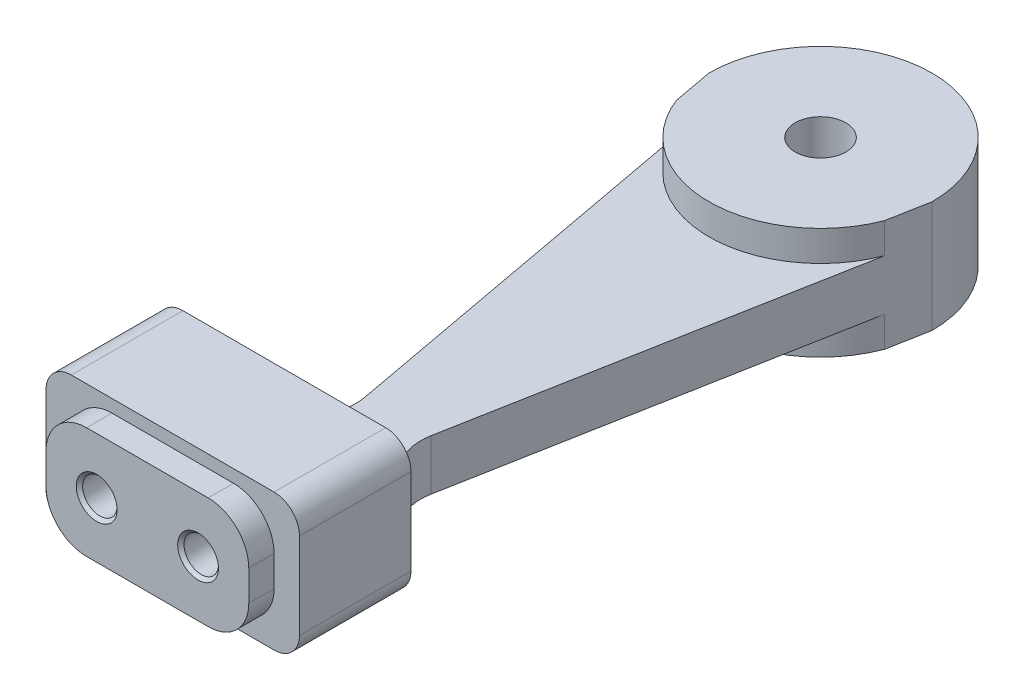
from build123d import *

# Parameters (mm, degrees)
BOSS_EXTRUDE1_DEPTH         = 22
BOSS_EXTRUDE2_DEPTH         = 5
BOSS_EXTRUDE3_DEPTH         = 5
SKETCH_4_3_2_R              = 5
BOSS_EXTRUDE4_DEPTH         = 11
M8_TAPPED_HOLE1_D           = 6.8
M8_TAPPED_HOLE1_DEPTH       = 19.957073895
M8_TAPPED_HOLE1_CSINK_D     = 8.05
M8_TAPPED_HOLE1_CSINK_ANGLE = 90
M8_TAPPED_HOLE1_TIP         = 2.042926105


with BuildPart() as part:
    # Sketch1 → Boss-Extrude1 (new body)
    with BuildSketch(Plane.XY):
        with BuildLine():
            Line((-20, -13.5), (20, -13.5))
            ThreePointArc((20, -13.5), (23.535533906, -12.035533906), (25, -8.5))
            Line((25, -8.5), (25, 8.5))
            ThreePointArc((25, 8.5), (23.535533906, 12.035533906), (20, 13.5))
            Line((20, 13.5), (-20, 13.5))
            ThreePointArc((-20, 13.5), (-23.535533906, 12.035533906), (-25, 8.5))
            Line((-25, 8.5), (-25, -8.5))
            ThreePointArc((-25, -8.5), (-23.535533906, -12.035533906), (-20, -13.5))
        make_face()
    extrude(amount=BOSS_EXTRUDE1_DEPTH)

    # Sketch2 → Boss-Extrude2 (add)
    with BuildSketch(Plane.XY.offset(22)):
        with BuildLine():
            Line((-12, -11), (12, -11))
            ThreePointArc((12, -11), (17.656854249, -8.656854249), (20, -3))
            Line((20, -3), (20, 3))
            ThreePointArc((20, 3), (17.656854249, 8.656854249), (12, 11))
            Line((12, 11), (-12, 11))
            ThreePointArc((-12, 11), (-17.656854249, 8.656854249), (-20, 3))
            Line((-20, 3), (-20, -3))
            ThreePointArc((-20, -3), (-17.656854249, -8.656854249), (-12, -11))
        make_face()
    extrude(amount=BOSS_EXTRUDE2_DEPTH)

    # Sketch 4_3 → Boss-Extrude3 (add, symmetric)
    with BuildSketch(Plane(origin=(0, 0, 0), x_dir=(1, 0, 0), z_dir=(0, 1, 0))):
        with BuildLine():
            ThreePointArc((31.338769383, 87.11590511), (23.260937212, 76.86922385), (10.8, 73))
            Line((10.8, 73), (10.8, 0))
            Line((10.8, 0), (25, 0))
            ThreePointArc((25, 0), (18.831156894, 4.245196236), (17.339679571, 11.583575604))
            Line((17.339679571, 11.583575604), (31.338769383, 87.11590511))
        make_face()
        with BuildLine():
            ThreePointArc((10.8, 73), (-1.660937212, 76.86922385), (-9.738769383, 87.11590511))
            Line((-9.738769383, 87.11590511), (4.260320429, 11.583575604))
            ThreePointArc((4.260320429, 11.583575604), (2.768843106, 4.245196236), (-3.4, 0))
            Line((-3.4, 0), (10.8, 0))
            Line((10.8, 0), (10.8, 73))
        make_face()
    extrude(amount=BOSS_EXTRUDE3_DEPTH, both=True)

    # Sketch 4_3 2 → Boss-Extrude4 (add, symmetric)
    with BuildSketch(Plane(origin=(0, 0, 0), x_dir=(1, 0, 0), z_dir=(0, 1, 0))):
        with BuildLine():
            ThreePointArc((32.8, 95), (10.8, 117), (-11.2, 95))
            Line((-11.2, 95), (-9.738769383, 87.11590511))
            ThreePointArc((-9.738769383, 87.11590511), (10.8, 73), (31.338769383, 87.11590511))
            Line((31.338769383, 87.11590511), (32.8, 95))
        make_face()
        with Locations(Location((10.8, 95, 0), (0, 0, 270))):
            Circle(SKETCH_4_3_2_R, mode=Mode.SUBTRACT)
    extrude(amount=BOSS_EXTRUDE4_DEPTH, both=True)

    # M8 Tapped Hole1
    with Locations(Plane(origin=(-10, 0, 27), x_dir=(1, 0, 0), z_dir=(0, 0, 1))):
        with Locations((0, 0), (20, 0)):
            CounterSinkHole(M8_TAPPED_HOLE1_D / 2, M8_TAPPED_HOLE1_CSINK_D / 2, depth=M8_TAPPED_HOLE1_DEPTH, counter_sink_angle=M8_TAPPED_HOLE1_CSINK_ANGLE)
            with Locations((0, 0, -(M8_TAPPED_HOLE1_DEPTH + M8_TAPPED_HOLE1_TIP / 2))):  # 118° drill point
                Cone(0, M8_TAPPED_HOLE1_D / 2, M8_TAPPED_HOLE1_TIP, mode=Mode.SUBTRACT)


solid = part.part
